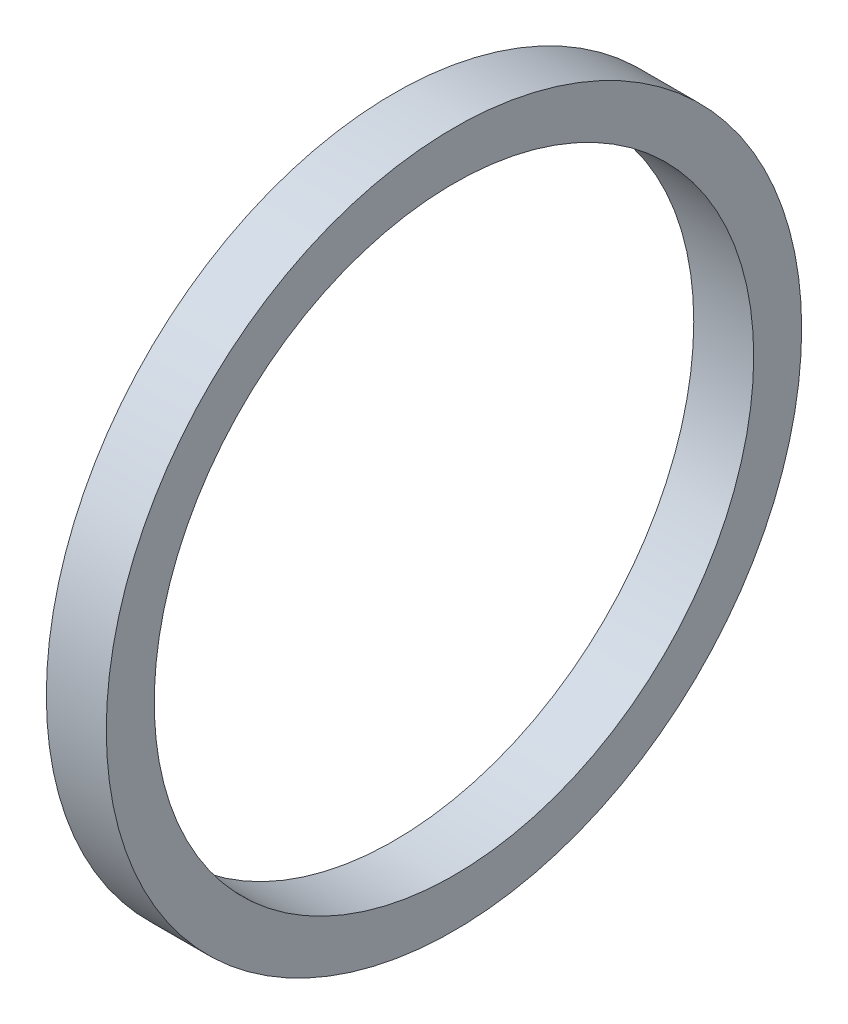
from build123d import *

# Parameters (mm, degrees)
SKETCH1_R           = 20.3
SKETCH1_R_2         = 17.5
BOSS_EXTRUDE1_DEPTH = 3.5


with BuildPart() as part:
    # Sketch1 → Boss-Extrude1 (new body)
    with BuildSketch(Plane(origin=(0, 0, 0), x_dir=(0, 0, -1), z_dir=(1, 0, 0))):
        Circle(SKETCH1_R)
        Circle(SKETCH1_R_2, mode=Mode.SUBTRACT)
    extrude(amount=BOSS_EXTRUDE1_DEPTH)


solid = part.part
